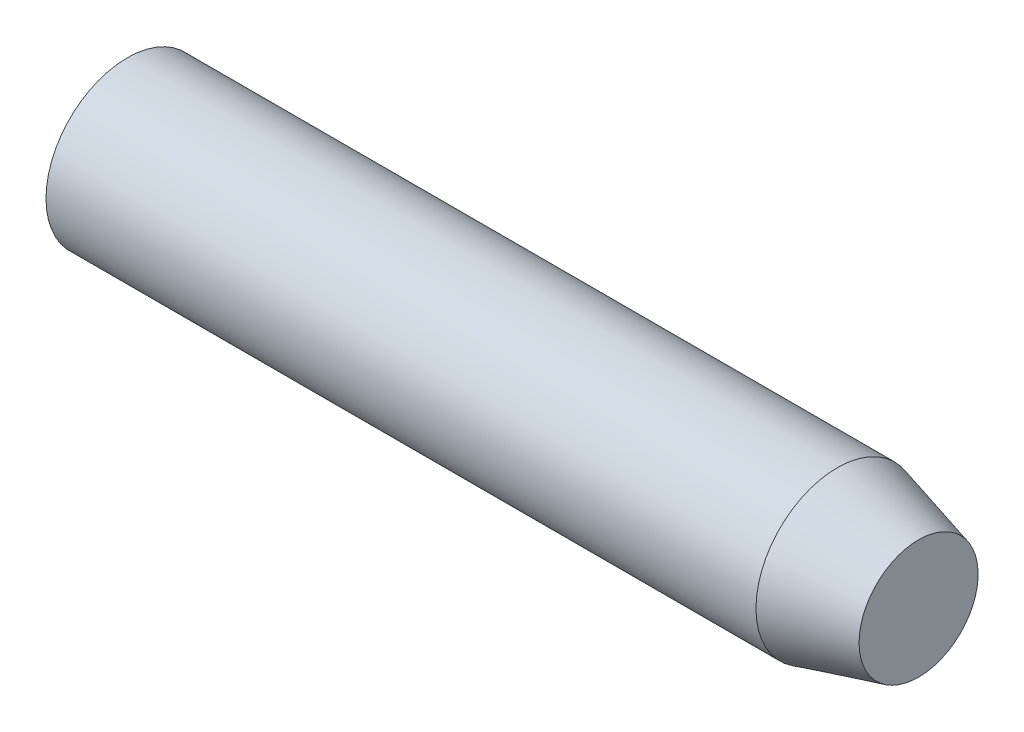
SolidWorks part; units mm, degrees
ref_plane "Front" through (0, 0, 0) normal (0, 0, 1) x (1, 0, 0)
ref_plane "Top" through (0, 0, 0) normal (0, 1, 0) x (1, 0, 0)
ref_plane "Right" through (0, 0, 0) normal (1, 0, 0) x (0, 0, -1)
sketch "Sketch1" plane through (0, 0, 0) normal (0, 1, 0) x (1, 0, 0)
  line L0 (-11.3907, 0) -> (1.7421, 0) construction
  line L1 (-1, -1) -> (0, -0.7321)
  line L2 (0, 0) -> (-10, 0)
  line L3 (0, 0) -> (0, -0.7321)
  line L4 (-1, -1) -> (-9.7321, -1)
  arc A0 (-10, 0) -> (-9.7321, -1) centre (-8, 0) ccw
  dimension "D2" = 4
  dimension "D1" = 2
  dimension "D3" = 1
  dimension "D4" = 15
  dimension "D5" = 10
revolve "Revolve1" add sketch "Sketch1" angle 360 mid plane about L0
